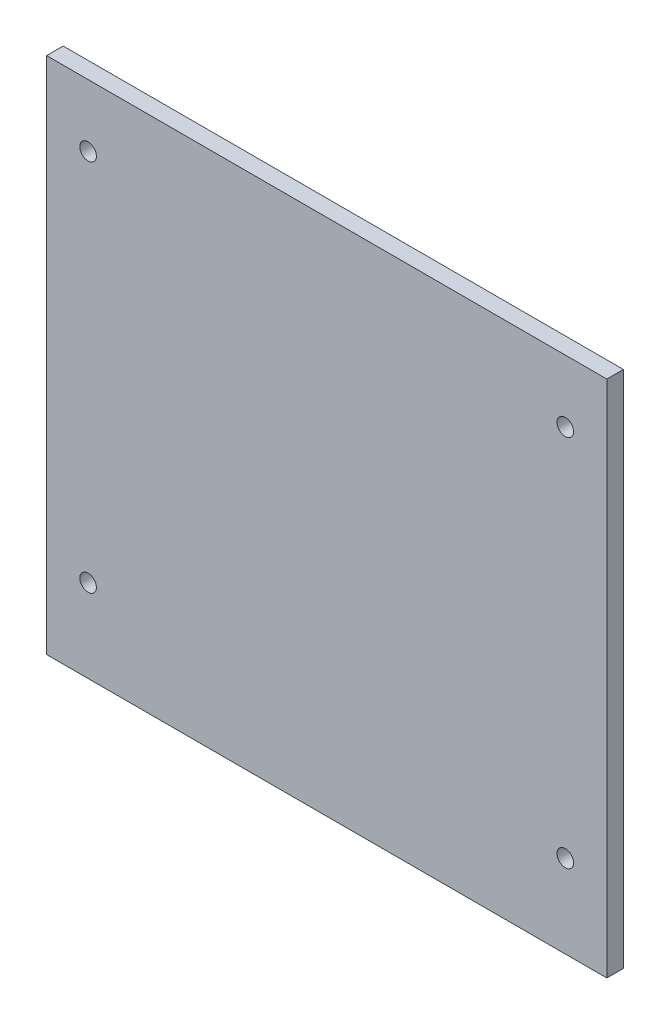
SolidWorks part; units mm, degrees
ref_plane "前视基准面" through (0, 0, 0) normal (0, 0, 1) x (1, 0, 0)
ref_plane "上视基准面" through (0, 0, 0) normal (0, 1, 0) x (1, 0, 0)
ref_plane "右视基准面" through (0, 0, 0) normal (1, 0, 0) x (0, 0, -1)
sketch "草图1" plane through (0, 0, 0) normal (0, 0, 1) x (1, 0, 0)
  line L0 (0, 0) -> (270, 0)
  line L1 (270, 0) -> (270, -250)
  line L2 (270, -250) -> (0, -250)
  line L3 (0, -250) -> (0, 0)
extrude "凸台-拉伸1" add sketch "草图1" along normal blind 8
sketch "草图2" plane through (0, 0, 8) normal (0, 0, 1) x (1, 0, 0)
  line L0 (270, -250) -> (250, -250)
  line L2 (0, -250) -> (270, -250) construction
  line L3 (250, -250) -> (250, -210)
  line L4 (250, -210) -> (250, -30)
  line L5 (250, -30) -> (20, -30)
  line L6 (20, -30) -> (20, -210)
  circle A0 centre (250, -30) radius 4
  circle A1 centre (250, -210) radius 4
  circle A2 centre (20, -210) radius 4
  circle A3 centre (20, -30) radius 4
extrude "切除-拉伸1" cut sketch "草图2" against normal blind 10
